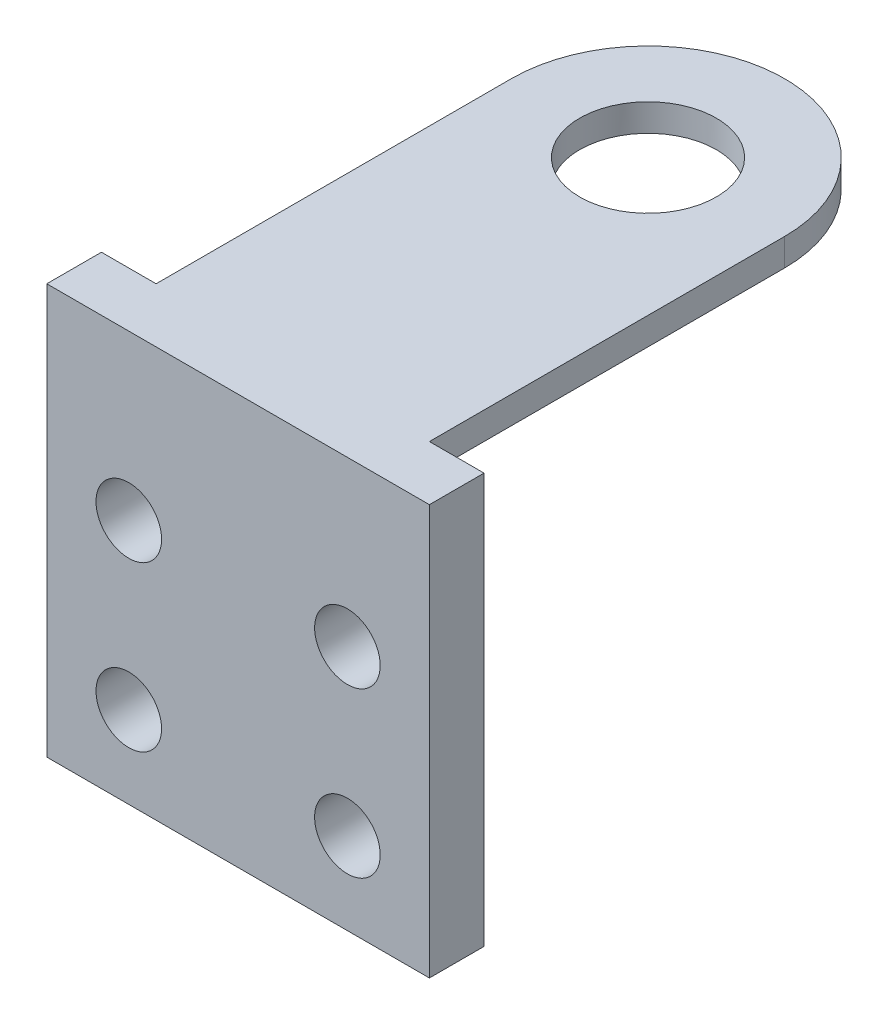
SolidWorks part; units mm, degrees
ref_plane "前视基准面" through (0, 0, 0) normal (0, 0, 1) x (1, 0, 0)
ref_plane "上视基准面" through (0, 0, 0) normal (0, 1, 0) x (1, 0, 0)
ref_plane "右视基准面" through (0, 0, 0) normal (1, 0, 0) x (0, 0, -1)
sketch "草图1" plane through (0, 0, 0) normal (0, 0, 1) x (1, 0, 0)
  line L1 (-15, 55) -> (55, 55)
  line L2 (-15, 55) -> (-15, -15)
  line L3 (-15, -15) -> (55, -15)
  line L4 (55, 55) -> (55, -15)
  circle A0 centre (0, 0) radius 6
  circle A1 centre (0, 30) radius 6
  circle A2 centre (40, 30) radius 6
  circle A3 centre (40, 0) radius 6
  dimension "D1" = 30
  dimension "D2" = 30
  dimension "D3" = 12
  dimension "D4" = 40
  dimension "D7" = 15
  dimension "D9" = 15
  dimension "D11" = 25
  dimension "D5" = 15
  dimension "D8" = 15
  dimension "D10" = 15
extrude "凸台-拉伸1" add sketch "草图1" along normal blind 10
sketch "草图2" plane through (0, 0, 10) normal (0, 0, 1) x (1, 0, 0)
  line L0 (55, -15) -> (55, 55) construction
  line L1 (-15, 55) -> (55, 55)
  line L2 (-15, 55) -> (-15, 60)
  line L3 (-15, 60) -> (55, 60)
  line L4 (55, 55) -> (55, 60)
extrude "凸台-拉伸2" add sketch "草图2" against normal blind 100
sketch "草图4" plane through (0, 60, 0) normal (0, 1, 0) x (1, 0, 0)
  line L0 (55, 90) -> (-15, 90) construction
  line L1 (-5, 65) -> (-5, 0)
  line L2 (45, 65) -> (45, 0)
  line L3 (45, 0) -> (78.5934, 0)
  line L4 (78.5934, 0) -> (78.5934, 103.7057)
  line L5 (78.5934, 103.7057) -> (-73.268, 103.7057)
  line L6 (-73.268, 103.7057) -> (-73.268, 50)
  line L7 (-5, 0) -> (-73.268, 0)
  line L8 (-15, 90) -> (-15, -10) construction
  line L10 (-73.268, 0) -> (-73.268, 50)
  circle A0 centre (20, 65) radius 12.5
  arc A1 (45, 65) -> (-5, 65) centre (20, 65) ccw
  dimension "D1" = 25
  dimension "D2" = 35
  dimension "D3" = 25
extrude "切除-拉伸1" cut sketch "草图4" against normal blind 10
